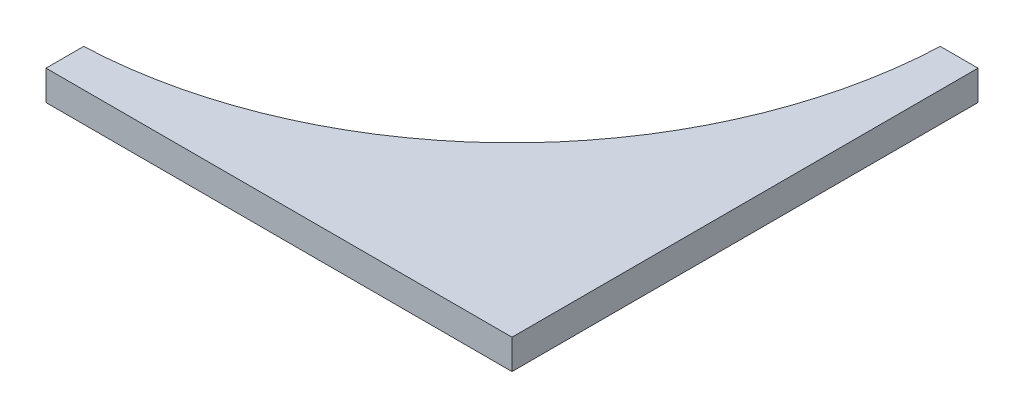
SolidWorks part; units mm, degrees
material "A3"
ref_plane "前视基准面" through (0, 0, 0) normal (0, 0, 1) x (1, 0, 0)
ref_plane "上视基准面" through (0, 0, 0) normal (0, 1, 0) x (1, 0, 0)
ref_plane "右视基准面" through (0, 0, 0) normal (1, 0, 0) x (0, 0, -1)
sketch "草图1" plane through (0, 0, 0) normal (0, 1, 0) x (1, 0, 0)
  line L0 (-125, 0) -> (0, 0)
  line L1 (0, 0) -> (0, 125)
  line L2 (0, 125) -> (-10.1042, 125)
  line L3 (-125, 0) -> (-125, 10.1042)
  arc A0 (-125, 10.1042) -> (-10.1042, 125) centre (-130, 130) ccw
  dimension "D2" = 120
  dimension "D1" = 125
  dimension "D3" = 5
  dimension "D4" = 5
extrude "凸台-拉伸1" add sketch "草图1" along normal blind 8
